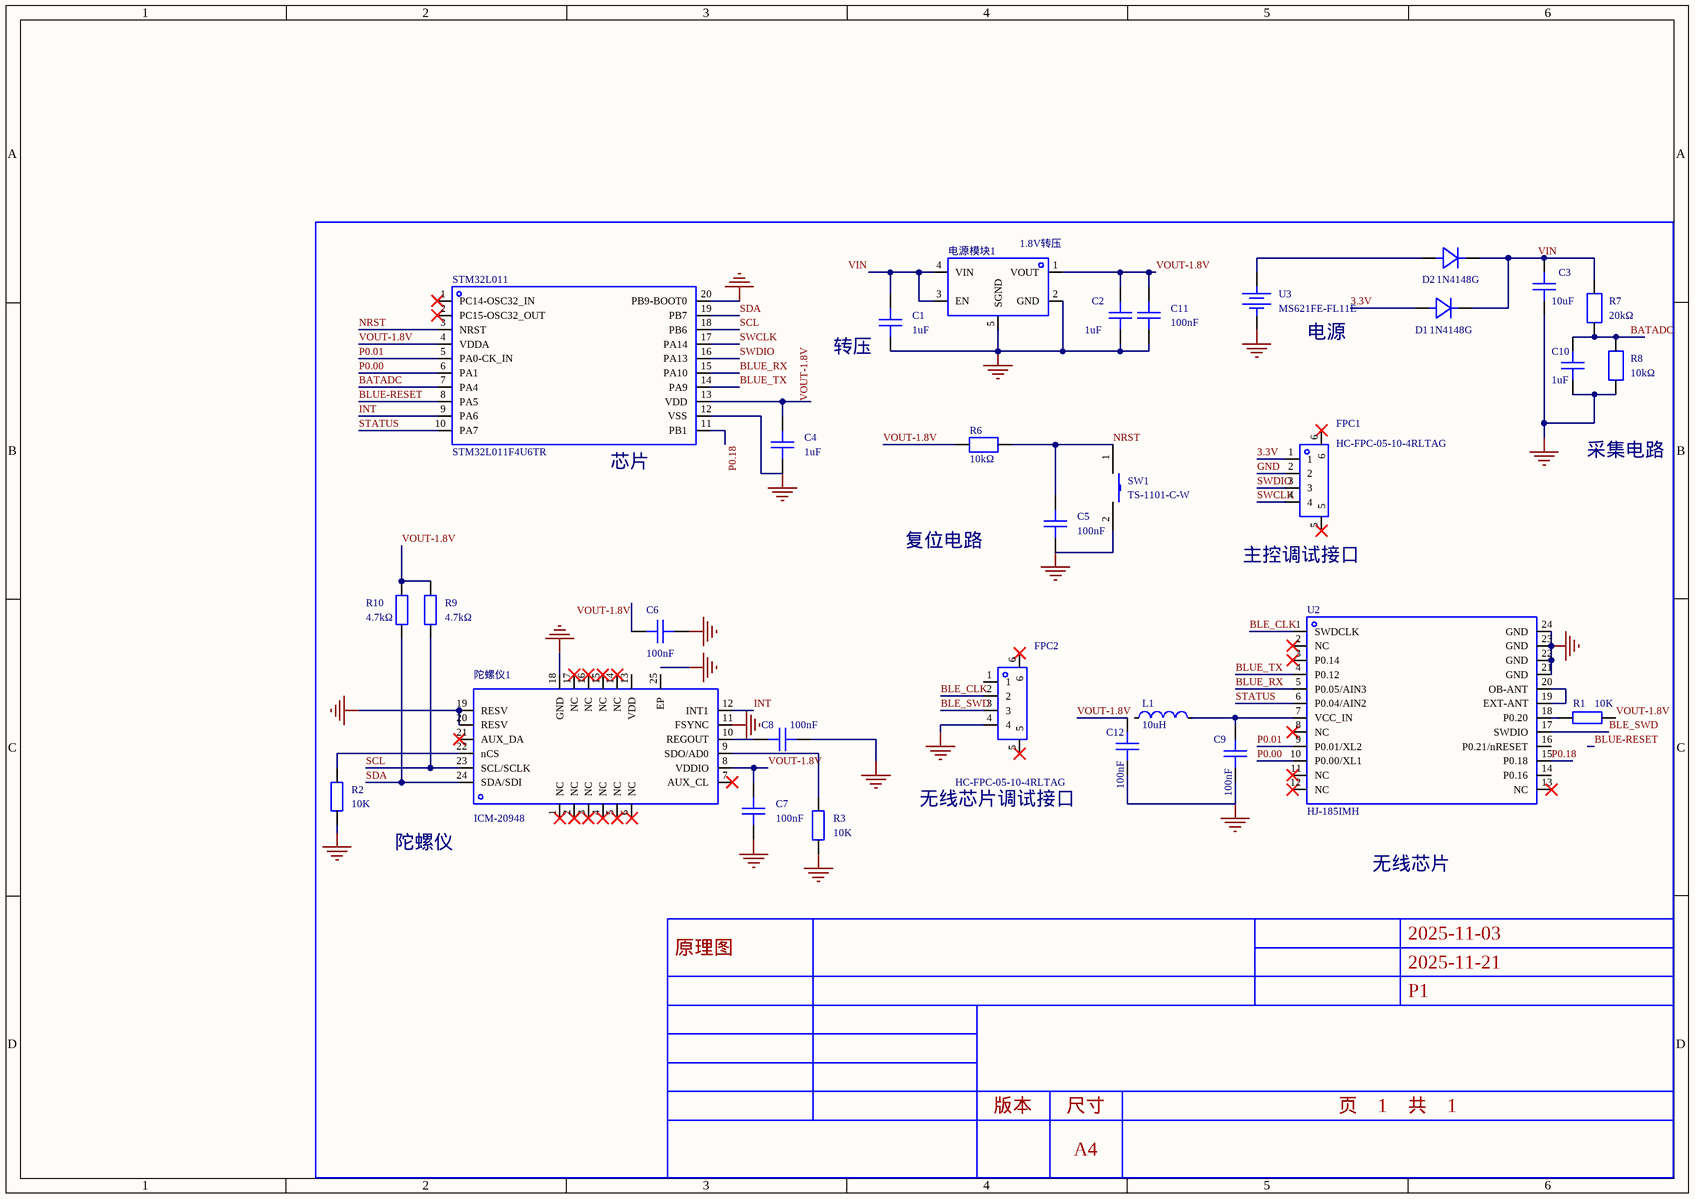
[diagram p0: MISC50958-3.schdoc]
# Altium project MISC50958-2.PrjPcb
1 sheet, 31 parts. Net scope: global (net labels, ports and power ports of the same name join across sheets).
Board file: MISC50958.pcbdoc

## Sheet MISC50958-3.schdoc
size 297 x 209 mm; Version: V1.0; @Project Name: MISC50958; @Page Count: 1; @Update Date: 2026-04-25; @Create Date: 2026-04-25; @Schematic Name: MISC50958; @Page No: 1; @Create Time: 06:47:21; @Update Time: 14:55:09; @Board Name: MISC50958

### Parts
C1  1uF  [C0402]
C2  1uF  [C0402]
C3  10uF  [C0805]
C4  1uF  [C0402]
C5  100nF  [C0402]
C6  100nF  [C0402]
C7  100nF  [C0402]
C8  100nF  [C0402]
C9  100nF  [C0402]
C10  1uF  [C0402]
C11  100nF  [C0603]
C12  100nF  [C0402]
D1  1N4148G  [SOD-723_L1.0-W0.6-P1.4-RD]
D2  1N4148G  [SOD-723_L1.0-W0.6-P1.4-RD]
FPC1  HC-FPC-05-10-4RLTAG  [FPC-SMD_4P-P0.50_HCTL_HC-FPC-05-10-4RLTAG]
FPC2  HC-FPC-05-10-4RLTAG  [FPC-SMD_4P-P0.50_HCTL_HC-FPC-05-10-4RLTAG]
L1  10uH  [L0603]
R1  10K  [R0603]
R2  10K  [R0603]
R3  10K  [R0603]
R6  10kΩ  [R0402]
R7  20kΩ  [R0402]
R8  10kΩ  [R0402]
R9  4.7kΩ  [R0402]
R10  4.7kΩ  [R0402]
STM32L011  STM32L011F4U6TR  [QFN-20_L3.0-W3.0-P0.50-BL]
SW1  TS-1101-C-W  [SW-SMD_L6.0-W3.3-LS8.0]
U2  HJ-185IMH  [LGA-24_L5.5-W5.0-P0.75-BL-EP]
U3  MS621FE-FL11E  [BAT-SMD_FL11E]
电源模块1  1.8V转压  [ZQFN-4L_L1.0-W1.0-P0.63-BL-EP]
陀螺仪1  ICM-20948  [QFN-24_L3.0-W3.0-P0.40-BL-EP]

### Nets
GND: C1.1 C2.1 C3.1 C4.1 C5.1 C6.1 C7.1 C8.2 C9.1 C10.1 C11.1 C12.1 FPC1.2 FPC2.4 R2.1 R3.1 R8.1 STM32L011.12(VSS) STM32L011.20(PB9-BOOT0) SW1.2 U2.21(GND) U2.22(GND) U2.23(GND) U2.24(GND) U3.2(-) 电源模块1.2(GND) 电源模块1.5(SGND) 陀螺仪1.11(FSYNC) 陀螺仪1.18(GND) 陀螺仪1.19(RESV) 陀螺仪1.20(RESV)
3.3V: D1.2(A) FPC1.1
BATADC: C10.2 R7.1 R8.2 STM32L011.7(PA4)
BLE_CLK: FPC2.2 U2.1(SWDCLK)
BLE_SWD: FPC2.3 U2.17(SWDIO)
BLUE-RESET: STM32L011.8(PA5)
BLUE_RX: STM32L011.15(PA10) U2.5(P0.05/AIN3)
BLUE_TX: STM32L011.14(PA9) U2.4(P0.12)
INT: STM32L011.9(PA6) 陀螺仪1.12(INT1)
NRST: C5.2 R6.2 STM32L011.3(NRST) SW1.1
P0.00: STM32L011.6(PA1) U2.10(P0.00/XL1)
P0.01: STM32L011.5(PA0-CK_IN) U2.9(P0.01/XL2)
P0.18: STM32L011.11(PB1) U2.15(P0.18)
SCL: R9.2 STM32L011.18(PB6) 陀螺仪1.23(SCL/SCLK)
SDA: R10.2 STM32L011.19(PB7) 陀螺仪1.24(SDA/SDI)
STATUS: STM32L011.10(PA7) U2.6(P0.04/AIN2)
SWCLK: FPC1.4 STM32L011.17(PA14)
SWDIO: FPC1.3 STM32L011.16(PA13)
VIN: C1.2 C3.2 D1.1(C) D2.1(C) R7.2 电源模块1.3(EN) 电源模块1.4(VIN)
VOUT-1.8V: C2.2 C4.2 C6.2 C7.2 C11.2 C12.2 R1.2 R6.1 R9.1 R10.1 STM32L011.4(VDDA) STM32L011.13(VDD) 电源模块1.1(VOUT) 陀螺仪1.8(VDDIO)
NetC8_1: C8.1 陀螺仪1.10(REGOUT)
NetC9_2: C9.2 L1.2 U2.7(VCC_IN)
NetD2_2: D2.2(A) U3.1(+)
NetR1_1: R1.1 U2.18(P0.20)
NetR2_2: R2.2 陀螺仪1.22(nCS)
NetR3_2: R3.2 陀螺仪1.9(SDO/AD0)
NetU2_19: U2.19(EXT-ANT) U2.20(OB-ANT)

Not connected (* = marked no-connect by the designer): FPC1 5* 6*; FPC2 1 5* 6*; L1 1; STM32L011 1(PC14-OSC32_IN)* 2(PC15-OSC32_OUT)*; U2 2(NC)* 3(P0.14)* 8(NC)* 11(NC)* 12(NC)* 13(NC)* 14(P0.16) 16(P0.21/nRESET); 陀螺仪1 1(NC)* 2(NC)* 3(NC)* 4(NC)* 5(NC)* 6(NC)* 7(AUX_CL)* 13(VDD) 14(NC)* 15(NC)* 16(NC)* 17(NC)* 21(AUX_DA)* 25(EP)

### Notes on the sheet
- (near C1) 转压
- (near U3) 电源
- 采集电路
- (near STM32L011) 芯片
- 复位电路
- (near FPC1) 主控调试接口
- 陀螺仪
- (near FPC2) 无线芯片调试接口
- 无线芯片
- 2025-11-03
- 原理图
- 2025-11-21
- P1
- 版本
- 尺寸
- A4
- 页    1    共    1

### Library data of the parts
C1 C2 C4 = CL05A105KA5NQNC: 容值:1uF;精度:±10%;额定电压:25V;温度系数:X5R;; Manufacturer: SAMSUNG(三星); AddInBom: yes; Tolerance: ±10%; Voltage Rating: 25V; Temperature Coefficient: X5R; ModelId: 36a51122f27c49738f86b3bfa98863e0; ModelName: C0402_L1.0-W0.5-H0.5; ModelTransform: 39.37,19.685,0,0,0,0,0,0,0; Device: CL05A105KA5NQNC; Symbol: CL05A105KA5NQNC; FootprintName: C0402; LCSC Part Name: 1uF ±10% 25V; SupplierPart: C52923; ManufacturerPart: CL05A105KA5NQNC; Supplier Footprint: 0402; JLCPCB Part Class: 基础库; Datasheet: https://item.szlcsc.com/datasheet/CL05A105KA5NQNC/53938.html; Supplier: LCSC; ConvertToPcb: yes; Value: 1uF
C3 = CGA0805X5R106K500MT: 容值:10uF;精度:±10%;额定电压:50V;温度系数:X5R;; Manufacturer: HRE(芯声); AddInBom: yes; Tolerance: ±10%; Voltage Rating: 50V; Temperature Coefficient: X5R; ModelId: 1ba041120af144c991958decab20d2410819f05c4eef4c71ace90d822a990e87; ModelName: C0805_L2.0-W1.3-H1.3; ModelTransform: 78.74,51.181,0,0,0,0,0,0.0005,0; Device: CGA0805X5R106K500MT; Symbol: CGA0805X5R106K500MT; FootprintName: C0805; LCSC Part Name: 10uF ±10% 50V; SupplierPart: C6119889; ManufacturerPart: CGA0805X5R106K500MT; Supplier Footprint: 0805; JLCPCB Part Class: Extended Part; Datasheet: https://item.szlcsc.com/datasheet/CGA0805X5R106K500MT/7062595.html; Supplier: LCSC; ConvertToPcb: yes; Value: 10uF
C5 C7-C9 = CL05B104KB54PNC: 容值:100nF;精度:±10%;额定电压:50V;温度系数:X7R;; Manufacturer: SAMSUNG(三星); AddInBom: yes; Tolerance: ±10%; Voltage Rating: 50V; Temperature Coefficient: X7R; ModelId: 36a51122f27c49738f86b3bfa98863e0; ModelName: C0402_L1.0-W0.5-H0.5; ModelTransform: 39.37,19.685,0,0,0,0,0,0,0; Device: CL05B104KB54PNC; Symbol: CL05B104KB54PNC; FootprintName: C0402; LCSC Part Name: 100nF ±10% 50V; SupplierPart: C307331; ManufacturerPart: CL05B104KB54PNC; Supplier Footprint: 0402; JLCPCB Part Class: 基础库; Datasheet: https://item.szlcsc.com/datasheet/CL05B104KB54PNC/291005.html; Supplier: LCSC; ConvertToPcb: yes; Value: 100nF
C6 = CL05B104KO5NNNC: 容值:100nF;精度:±10%;额定电压:16V;温度系数:X7R;; Manufacturer: SAMSUNG(三星); AddInBom: yes; Tolerance: ±10%; Voltage Rating: 16V; Temperature Coefficient: X7R; ModelId: 36a51122f27c49738f86b3bfa98863e0; ModelName: C0402_L1.0-W0.5-H0.5; ModelTransform: 39.37,19.685,0,0,0,0,0,0,0; Device: CL05B104KO5NNNC; Symbol: CL05B104KO5NNNC; FootprintName: C0402; LCSC Part Name: 100nF ±10% 16V; SupplierPart: C1525; ManufacturerPart: CL05B104KO5NNNC; Supplier Footprint: 0402; JLCPCB Part Class: 基础库; Datasheet: https://item.szlcsc.com/datasheet/CL05B104KO5NNNC/1877.html; Supplier: LCSC; ConvertToPcb: yes; Value: 100nF
C10 = CL05A105KA5NQNC: 容值:1uF;精度:±10%;额定电压:25V;温度系数:X5R;; Manufacturer: SAMSUNG(三星); 3D Model: 36a51122f27c49738f86b3bfa98863e0; 3D Model Transform: 39.37,19.685,0,0,0,0,0,0,0; Tolerance: ±10%; Voltage Rating: 25V; Temperature Coefficient: X5R; AddInBom: yes; ModelName: C0402_L1.0-W0.5-H0.5; Device: CL05A105KA5NQNC; Symbol: CL05A105KA5NQNC; LCSC Part Name: 1uF ±10% 25V; Supplier Part: C52923; Manufacturer Part: CL05A105KA5NQNC; Supplier Footprint: 0402; JLCPCB Part Class: 基础库; Datasheet: https://item.szlcsc.com/datasheet/CL05A105KA5NQNC/53938.html; Supplier: LCSC; Value: 1uF; FootprintName: C0402; ConvertToPcb: yes
C11 = CGA0603X7R104K500JT: 容值:100nF;精度:±10%;额定电压:50V;温度系数:X7R;; Manufacturer: HRE(芯声); AddInBom: yes; Tolerance: ±10%; Voltage Rating: 50V; Temperature Coefficient: X7R; ModelId: ac125912035d415993ca9572d50418b10819f05c4eef4c71ace90d822a990e87; ModelName: C0603_L1.6-W0.8-H0.8; ModelTransform: 62.992,31.496,0,0,0,0,0,0,0; Device: CGA0603X7R104K500JT; Symbol: CGA0603X7R104K500JT; FootprintName: C0603; LCSC Part Name: 100nF ±10% 50V; SupplierPart: C6119867; ManufacturerPart: CGA0603X7R104K500JT; Supplier Footprint: 0603; JLCPCB Part Class: Extended Part; Datasheet: https://item.szlcsc.com/datasheet/CGA0603X7R104K500JT/7062573.html; Supplier: LCSC; ConvertToPcb: yes; Value: 100nF
C12 = CL05B104KB54PNC: 容值:100nF;精度:±10%;额定电压:50V;温度系数:X7R;; Manufacturer: SAMSUNG(三星); 3D Model: 36a51122f27c49738f86b3bfa98863e0; 3D Model Transform: 39.37,19.685,0,0,0,0,0,0,0; Tolerance: ±10%; Voltage Rating: 50V; Temperature Coefficient: X7R; AddInBom: yes; ModelName: C0402_L1.0-W0.5-H0.5; Device: CL05B104KB54PNC; Symbol: CL05B104KB54PNC; LCSC Part Name: 100nF ±10% 50V; Supplier Part: C307331; Manufacturer Part: CL05B104KB54PNC; Supplier Footprint: 0402; JLCPCB Part Class: 基础库; Datasheet: https://item.szlcsc.com/datasheet/CL05B104KB54PNC/291005.html; Supplier: LCSC; Value: 100nF; FootprintName: C0402; ConvertToPcb: yes
D1 = 1N4148G: 正向压降(Vf):1.25V@150mA;直流反向耐压(Vr):100V;整流电流:150mA;反向恢复时间(Trr):4ns;; Manufacturer: GOODWORK(固得沃克); AddInBom: yes; Voltage - DC Reverse(Vr): 100V; Current - Rectified: 150mA; Pd - Power Dissipation: 210mW; Reverse Leakage Current (Ir): 1uA; Reverse Recovery Time (trr): 4ns; Non-Repetitive Peak Forward Surge Current: 2A; ModelId: 93ee04c805894507a1c6d2f169bb13b7; ModelTransform: 55.118,23.622,0,0,0,0,0.005,0,0; Device: 1N4148G; Symbol: 1N4148G; FootprintName: SOD-723_L1.0-W0.6-P1.4-RD; LCSC Part Name: 1N4148G; SupplierPart: C42429389; ManufacturerPart: 1N4148G; Supplier Footprint: SOD-723; JLCPCB Part Class: 扩展库; Datasheet: https://item.szlcsc.com/datasheet/1N4148G/44451528.html; Supplier: LCSC; ConvertToPcb: yes; Voltage - Forward(Vf@If): 1.25V@150mA; ModelName: SOD-723_L1.0-W0.6-P1.4-RD
D2 = 1N4148G: 正向压降(Vf):1.25V@150mA;直流反向耐压(Vr):100V;整流电流:150mA;反向恢复时间(Trr):4ns;; Manufacturer: GOODWORK(固得沃克); 3D Model: 93ee04c805894507a1c6d2f169bb13b7; 3D Model Transform: 55.118,23.622,0,0,0,0,0.005,0,0; Voltage - DC Reverse(Vr): 100V; Current - Rectified: 150mA; Pd - Power Dissipation: 210mW; Reverse Leakage Current (Ir): 1uA; Reverse Recovery Time (trr): 4ns; Non-Repetitive Peak Forward Surge Current: 2A; AddInBom: yes; Device: 1N4148G; Symbol: 1N4148G; LCSC Part Name: 1N4148G; Supplier Part: C42429389; Manufacturer Part: 1N4148G; Supplier Footprint: SOD-723; JLCPCB Part Class: 扩展库; Datasheet: https://item.szlcsc.com/datasheet/1N4148G/44451528.html; Supplier: LCSC; Voltage - Forward(Vf@If): 1.25V@150mA; FootprintName: SOD-723_L1.0-W0.6-P1.4-RD; ConvertToPcb: yes; ModelName: SOD-723_L1.0-W0.6-P1.4-RD
FPC1 = HC-FPC-05-10-4RLTAG: 锁定特性:翻盖式;触点类型:下接;触点数量:4P;间距:0.5mm;安装方式:卧贴;工作温度:-55℃~+85℃;; Manufacturer: HCTL(华灿天禄); AddInBom: yes; Locking Feature: 翻盖式; Number of Contacts: 4P; Pitch: 0.5mm; FFC, FCB Thickness: 0.3mm; ModelId: a1d39e444eed49619ec61cdfde0f08d4; ModelTransform: 148.8186,154.33,0,0,0,0,0,17.716,0; Device: HC-FPC-05-10-4RLTAG; Symbol: HC-FPC-05-10-4RLTAG; FootprintName: FPC-SMD_4P-P0.50_HCTL_HC-FPC-05-10-4RLTAG; LCSC Part Name: 翻盖式 下接 P数:4P 间距:0.5mm; SupplierPart: C5213727; ManufacturerPart: HC-FPC-05-10-4RLTAG; Supplier Footprint: SMD,P=0.5mm,卧贴; JLCPCB Part Class: 扩展库; Datasheet: https://item.szlcsc.com/datasheet/HC-FPC-05-10-4RLTAG/5909019.html; Supplier: LCSC; ConvertToPcb: yes; Contact Type: 下接; Mounting Type: 卧贴; Height Above Board: 1mm; Contact Material: 铜合金; Operating Temperature: -55℃~+85℃; ModelName: FPC-SMD_4P-P0.50_HCTL_HC-FPC-05-10-4RLTAG
FPC2 = HC-FPC-05-10-4RLTAG: 锁定特性:翻盖式;触点类型:下接;触点数量:4P;间距:0.5mm;安装方式:卧贴;工作温度:-55℃~+85℃;; Manufacturer: HCTL(华灿天禄); 3D Model: a1d39e444eed49619ec61cdfde0f08d4; 3D Model Transform: 148.8186,154.33,0,0,0,0,0,17.716,0; Locking Feature: 翻盖式; Number of Contacts: 4P; Pitch: 0.5mm; FFC, FCB Thickness: 0.3mm; AddInBom: yes; Device: HC-FPC-05-10-4RLTAG; Symbol: HC-FPC-05-10-4RLTAG; LCSC Part Name: 翻盖式 下接 P数:4P 间距:0.5mm; Supplier Part: C5213727; Manufacturer Part: HC-FPC-05-10-4RLTAG; Supplier Footprint: SMD,P=0.5mm,卧贴; JLCPCB Part Class: 扩展库; Datasheet: https://item.szlcsc.com/datasheet/HC-FPC-05-10-4RLTAG/5909019.html; Supplier: LCSC; Contact Type: 下接; Mounting Type: 卧贴; Height Above Board: 1mm; Contact Material: 铜合金; Operating Temperature: -55℃~+85℃; FootprintName: FPC-SMD_4P-P0.50_HCTL_HC-FPC-05-10-4RLTAG; ConvertToPcb: yes; ModelName: FPC-SMD_4P-P0.50_HCTL_HC-FPC-05-10-4RLTAG
L1 = L_0603: Symbol: SDFL1608S100KTF; AddInBom: yes; ModelId: 2bc5ec593d464d6ba9807aec0b5673c20819f05c4eef4c71ace90d822a990e87; ModelName: L0603_L1.6-W0.8-H0.5_BEAD; ModelTransform: 62.992,31.496,0,180,0,0,0.094,0.629,0; Device: L_0603; FootprintName: L0603; Supplier Footprint: L0603; ConvertToPcb: yes; Value: 10uH
R1-R3 = Res_0603: Symbol: 电阻; ConvertToPcb: yes; ModelId: fc143cca1e79419f9cd78b61e9279f080819f05c4eef4c71ace90d822a990e87; ModelTransform: 31.8897,63.7794,0,90,0,0,0,0,0; Device: Res_0603; FootprintName: R0603; AddInBom: yes; Supplier Footprint: 0603; Value: 10K; ModelName: R0603
R6 R8 = AS0210KF: 阻值:10kΩ;精度:±1%;功率:62.5mW;工作电压:50V;温度系数:±200ppm/℃;; Manufacturer: HKR(香港电阻); AddInBom: yes; Tolerance: ±1%; Power(Watts): 62.5mW; Voltage-Supply(Max): 50V; ModelId: 98c88bc2b9094f218f3a3e30a7012738; ModelName: R0402_L1.0-W0.5-H0.4; ModelTransform: 39.37,19.685,0,0,0,0,0,0,0; Device: AS0210KF; Symbol: AS0210KF; FootprintName: R0402; LCSC Part Name: 10K ±1%; SupplierPart: C49330233; ManufacturerPart: AS0210KF; Supplier Footprint: 0402; JLCPCB Part Class: 扩展库; Datasheet: https://item.szlcsc.com/datasheet/AS0210KF/51811997.html; Supplier: LCSC; ConvertToPcb: yes; Value: 10kΩ; Temperature Coefficient: ±200ppm/℃; Operating Temperature: -55℃~+155℃
R7 = FRQ0402F2002TS: 电阻类型:厚膜电阻;阻值:20kΩ;精度:±1%;功率:62.5mW;工作电压:50V;温度系数:±100ppm/℃;; Manufacturer: FOJAN(富捷); AddInBom: yes; Tolerance: ±1%; Power(Watts): 62.5mW; Voltage-Supply(Max): 50V; ModelId: 98c88bc2b9094f218f3a3e30a7012738; ModelName: R0402_L1.0-W0.5-H0.4; ModelTransform: 39.37,19.685,0,0,0,0,0,0,0; Device: FRQ0402F2002TS; Symbol: FRQ0402F2002TS; FootprintName: R0402; LCSC Part Name: 厚膜电阻 0402 20KΩ ±1% 62.5mW; SupplierPart: C49196870; ManufacturerPart: FRQ0402F2002TS; Supplier Footprint: 0402; JLCPCB Part Class: 扩展库; Datasheet: https://item.szlcsc.com/datasheet/FRQ0402F2002TS/51599118.html; Supplier: LCSC; ConvertToPcb: yes; Type: 厚膜电阻; Value: 20kΩ; Temperature Coefficient: ±100ppm/℃; Operating Temperature: -55℃~+155℃
R9 R10 = 0402WGF4701TCE: 电阻类型:厚膜电阻;阻值:4.7kΩ;精度:±1%;功率:62.5mW;工作电压:50V;温度系数:±100ppm/℃;; Manufacturer: UNI-ROYAL(厚声); AddInBom: yes; Tolerance: ±1%; Power(Watts): 62.5mW; Voltage-Supply(Max): 50V; ModelId: 98c88bc2b9094f218f3a3e30a7012738; ModelName: R0402_L1.0-W0.5-H0.4; ModelTransform: 39.37,19.685,0,0,0,0,0,0,0; Device: 0402WGF4701TCE; Symbol: 0402WGF4701TCE; FootprintName: R0402; LCSC Part Name: 4.7kΩ ±1% 62.5mW 厚膜电阻; SupplierPart: C25900; ManufacturerPart: 0402WGF4701TCE; Supplier Footprint: 0402; JLCPCB Part Class: 基础库; Datasheet: https://item.szlcsc.com/datasheet/0402WGF4701TCE/26643.html; Supplier: LCSC; ConvertToPcb: yes; Type: 厚膜电阻; Value: 4.7kΩ; Temperature Coefficient: ±100ppm/℃; Operating Temperature: -55℃~+155℃
STM32L011 = STM32L011F4U6TR: CPU内核:ARM-M系列;CPU最大主频:32MHz;应用领域:-;; Manufacturer: ST(意法半导体); AddInBom: yes; CPU Maximum Speed: 32MHz; Program Storage Size: 16KB; Number of I/O: 16; ADC (Bit): 12bit; Voltage - Supply: 1.65V~3.6V; ModelId: 3315b776f0c445e28586e7f5f0ae1c1c; ModelName: QFN-20_L3.0-W3.0-H0.6-P0.50-BL; ModelTransform: 118.11,118.11,0,180,0,0,0.027,0.002,0; Device: STM32L011F4U6TR; Symbol: STM32L011F4U6TR; FootprintName: QFN-20_L3.0-W3.0-P0.50-BL; LCSC Part Name: 超低功耗Arm Cortex-M0+ MCU，具有16-KB Flash存储器和32 MHz CPU; SupplierPart: C329283; ManufacturerPart: STM32L011F4U6TR; Supplier Footprint: UFQFPN-20(3x3); JLCPCB Part Class: Extended Part; Datasheet: https://item.szlcsc.com/datasheet/STM32L011F4U6TR/308908.html; Supplier: LCSC; ConvertToPcb: yes; CPU Core: ARM-M系列; Applications: -
SW1 = TS-1101-C-W: 电路结构:单刀单掷;按钮形状:矩形按钮;作用力:260gf;安装方式:立贴;开关长度:6mm;开关宽度:3.6mm;开关高度:2.5mm;带支架:不带;触点电流:50mA;额定电压(AC):-;额定电压(DC):12V;额定功率:-;绝缘电阻:-;带灯:无;机械寿命:5万次;; Manufacturer: XKB Connectivity(中国星坤); AddInBom: yes; Circuit: 单刀单掷; Actuator Style: 矩形按钮; Operating Force: 260gf; Switch Length: 6mm; Switch Width: 3.6mm; Switch Height: 2.5mm; Strike Gundam: 不带; Contact Current: 50mA; Voltage Rating (DC): 12V; Actuator/Cap Color: 白色带淡绿; With Lamp: 无; Mechanical Life: 5万次; ModelId: b2f4ea9f0afc4b0786d53dba66ceb9e40819f05c4eef4c71ace90d822a990e87; ModelName: SW-SMD_L6.0-W3.3-H5-LS8.0; ModelTransform: 314.96,129.921,0,0,0,0,0,0,0; Device: TS-1101-C-W; Symbol: TS-1101-C-W; FootprintName: SW-SMD_L6.0-W3.3-LS8.0; LCSC Part Name: 6*3.6*2.5mm 立贴 轻触开关; SupplierPart: C318938; ManufacturerPart: TS-1101-C-W; Supplier Footprint: SMD; JLCPCB Part Class: Extended Part; Datasheet: https://atta.szlcsc.com/upload/public/pdf/source/20200227/C318938_C2E53B1EEDE37D980A33616AC086DE53.pdf; Supplier: LCSC; ConvertToPcb: yes; Mounting Style: 立贴; Voltage Rating (AC): -; Power Rating: -; Insulation Resistance: -; IP Rating: -; Pin Style: -; Operating Temperature: -30℃~+85℃
U2 = HJ-185IMH: Manufacturer: HongJia(宏佳); AddInBom: yes; ModelId: 59bc6a2971be44d9887f8cef0a91210f; ModelTransform: 216.535,197.2437,0,0,0,0,0,0,0; Device: HJ-185IMH; Symbol: HJ-185IMH; FootprintName: LGA-24_L5.5-W5.0-P0.75-BL-EP; LCSC Part Name: HJ-185IMH; SupplierPart: C2931605; ManufacturerPart: HJ-185IMH; Supplier Footprint: LGA-24(5x5.5); JLCPCB Part Class: 扩展库; Datasheet: https://atta.szlcsc.com/upload/public/pdf/source/20211228/482222A794A9EC338B2F62A7A7961019.pdf; Supplier: LCSC; ConvertToPcb: yes; ModelName: LGA-24_L5.5-W5.0-P0.75-BL-EP
U3 = MS621FE-FL11E: 标称电压:3V;; Manufacturer: Seiko(精工); AddInBom: yes; nominal voltage: 3V; Capacity: 5.5mAh; Chemical system: 锂离子; Battery Rechargeability: 可充电; unit: 1个; ModelId: 2a91895ee9794bf0b802e980dc7ffaa7; ModelName: CAP-SMD_FL11E; ModelTransform: 366.141,267.716,0,0,0,0,-146.969,0,0; Device: MS621FE-FL11E; Symbol: MS621FE-FL11E; FootprintName: BAT-SMD_FL11E; LCSC Part Name: Seiko(精工) 锂离子电池 3V 5.5mAh 1个; SupplierPart: C80909; ManufacturerPart: MS621FE-FL11E; Supplier Footprint: -; JLCPCB Part Class: 扩展库; Datasheet: https://item.szlcsc.com/datasheet/MS621FE-FL11E/82059.html; Supplier: LCSC; ConvertToPcb: yes; diameter: 6.8mm; thickness: 2.2mm; Type: 电池; Type of electrolyte: -
电源模块1 = RT9073A-18GQZ: 输出类型:固定;工作电压:5.5V;输出电压:1.8V;输出电流:250mA;电源纹波抑制比(PSRR):75dB@(1kHz);输出极性:正极;; Manufacturer: RICHTEK(立锜); AddInBom: yes; Output Type: 固定; Voltage - Supply: 5.5V; Output Voltage: 1.8V; Output Current: 250mA; Voltage Dropout: 680mV@(250mA); standby current: 1uA; Noise: 48uVrms; Output Configuration: 正极; Number of Outputs: 1; ModelId: 8cc83e0407be4bc0bfb8d0f677574aff; ModelName: ZQFN-4L_L1.0-W1.0-H0.4-P0.63-BL-EP; ModelTransform: 39.37,39.37,0,90,0,0,0,0,0; Device: RT9073A-18GQZ; Symbol: RT9073A-18GQZ; Manufacturer Part: 1.8V转压; FootprintName: ZQFN-4L_L1.0-W1.0-P0.63-BL-EP; LCSC Part Name: 输入5.5V 输出1.8V 250mA; SupplierPart: C250431; Supplier Footprint: ZQFN-4L-EP(1x1); JLCPCB Part Class: 扩展库; Datasheet: https://item.szlcsc.com/datasheet/RT9073A-18GQZ/246459.html; Supplier: LCSC; ConvertToPcb: yes; Power Supply Rejection Ratio (PSRR): 75dB@(1kHz); Features: 过热保护；过流保护; Operating Temperature: -40℃~+85℃@(Ta)
陀螺仪1 = ICM-20948: 传感器类型:加速度计陀螺仪;接口类型:I2C；SPI;; Manufacturer: TDK InvenSense(应美盛); AddInBom: yes; Accelerometer Sensing Axis: X,Y,Z; Acceleration Measurement Range (MAX): ±16g; Gyroscope Measurement Range (MAX): ±2000dps; Output Bits: 16bit; Voltage - Supply: 1.71V~3.6V; Cache Size: 0.5KB; Standby Current: 8uA; ModelId: b6102d6ded464b998bbf3859d0a01637; ModelName: QFN-24_L3.0-W3.0-H0.9-P0.40-BL-EP; ModelTransform: 118.11,118.11,0,90,0,0,0,0,0; Device: ICM-20948; Symbol: ICM-20948; FootprintName: QFN-24_L3.0-W3.0-P0.40-BL-EP; LCSC Part Name: 九轴MEMS运动追踪器件; SupplierPart: C726001; ManufacturerPart: ICM-20948; Supplier Footprint: QFN-24(3x3); JLCPCB Part Class: 扩展库; Datasheet: https://item.szlcsc.com/datasheet/ICM-20948/772651.html; Supplier: LCSC; ConvertToPcb: yes; Gyroscope Sensing Axis: X,Y,Z; Sensor Type: 加速度计陀螺仪; Interface: I2C；SPI; Operating Temperature: -40℃~+85℃